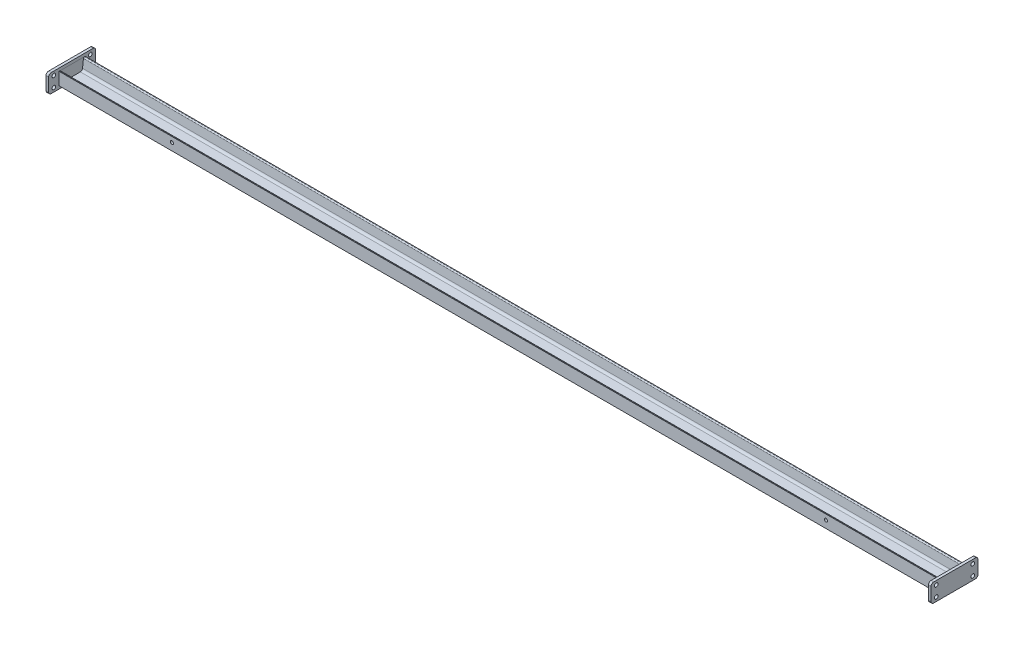
from build123d import *

# Parameters (mm, degrees)
GB_T707_1988_HOT_ROLLED_CHANNEL_10_1_DEPTH = 3371
SKETCH3_R                                  = 7
BOSS_EXTRUDE1_DEPTH                        = 10
SKETCH9_R                                  = 6
CUT_EXTRUDE1_DEPTH                         = 10


with BuildPart() as part:
    # Sketch13 → Gb／t707-1988 Hot-Rolled Channel 10(1) (new body)
    with BuildSketch(Plane(origin=(-1685.5, 0, -50), x_dir=(0, 1, 0), z_dir=(1, 0, 0))):
        with BuildLine():
            Line((48, 100), (0, 100))
            Line((0, 100), (0, 0))
            Line((0, 0), (48, 0))
            Line((48, 0), (48, 2.474327591))
            ThreePointArc((48, 2.474327591), (46.921208267, 5.284676138), (44.239019546, 6.651319552))
            Line((44.239019546, 6.651319552), (12.911508062, 9.943973689))
            ThreePointArc((12.911508062, 9.943973689), (7.483268983, 12.709799645), (5.3, 18.397409799))
            Line((5.3, 18.397409799), (5.3, 81.602590201))
            ThreePointArc((5.3, 81.602590201), (7.483268983, 87.290200355), (12.911508062, 90.056026311))
            Line((12.911508062, 90.056026311), (44.239019546, 93.348680448))
            ThreePointArc((44.239019546, 93.348680448), (46.921208267, 94.715323862), (48, 97.525672409))
            Line((48, 97.525672409), (48, 100))
        make_face()
    extrude(amount=GB_T707_1988_HOT_ROLLED_CHANNEL_10_1_DEPTH)

    # Sketch9 → Cut-Extrude1 (cut)
    with BuildSketch(Plane(origin=(0, 0, 50), x_dir=(-1, 0, 0), z_dir=(0, 0, -1))):
        with Locations(Location((-1253, 28, 0), (0, 0, 90))):
            Circle(SKETCH9_R)
        with Locations(Location((1253, 28, 0), (0, 0, 90))):
            Circle(SKETCH9_R)
    extrude(amount=CUT_EXTRUDE1_DEPTH, mode=Mode.SUBTRACT)


with BuildPart() as body_2:
    # Sketch3 → Boss-Extrude1 (new body)
    with BuildSketch(Plane.ZY.offset(1685.5)):
        with BuildLine():
            Line((-80, 59), (80, 59))
            ThreePointArc((80, 59), (87.071067812, 56.071067812), (90, 49))
            Line((90, 49), (90, -1))
            ThreePointArc((90, -1), (87.071067812, -8.071067812), (80, -11))
            Line((80, -11), (-80, -11))
            ThreePointArc((-80, -11), (-87.071067812, -8.071067812), (-90, -1))
            Line((-90, -1), (-90, 49))
            ThreePointArc((-90, 49), (-87.071067812, 56.071067812), (-80, 59))
        make_face()
        with Locations((-70, 44)):
            Circle(SKETCH3_R, mode=Mode.SUBTRACT)
        with Locations(Location((-70, 4, 0), (0, 0, 180))):
            Circle(SKETCH3_R, mode=Mode.SUBTRACT)
        with Locations((70, 4)):
            Circle(SKETCH3_R, mode=Mode.SUBTRACT)
        with Locations(Location((70, 44, 0), (0, 0, 180))):
            Circle(SKETCH3_R, mode=Mode.SUBTRACT)
    extrude(amount=BOSS_EXTRUDE1_DEPTH)


with BuildPart() as body_3:
    # Mirror3: mirrored copy
    add(body_2.part.mirror(Plane(origin=(0, 0, 0), x_dir=(0, 0, 1), z_dir=(1, 0, 0))))


solid = Compound([part.part, body_2.part, body_3.part])
